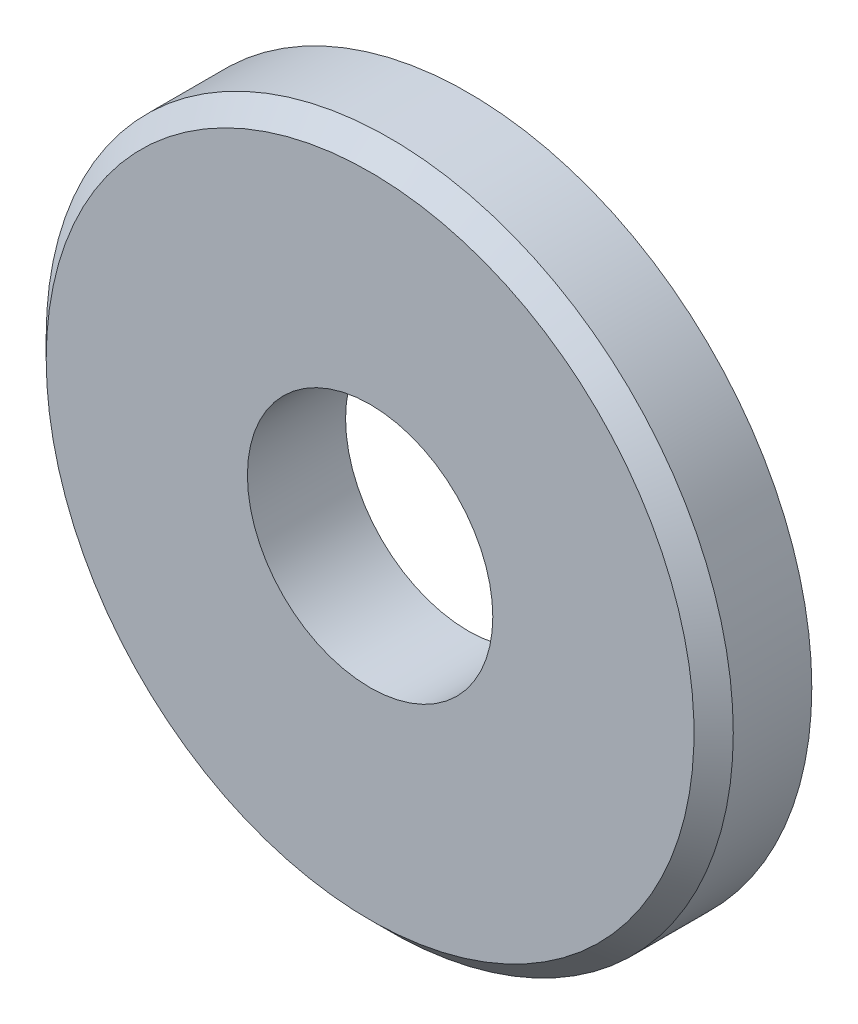
from build123d import *


with BuildPart() as part:
    # 草图1 → 旋转1 (revolve)
    with BuildSketch(Plane.XZ, mode=Mode.PRIVATE) as revolve_1_sk:
        Polygon((6.25, 2.5), (6.25, -2.5), (17.5, -2.5), (17.5, 1.5), (16.5, 2.5), align=None)
    revolve(revolve_1_sk.sketch.rotate(Axis((0, 0, 2.5), (0, 0, -1)), 180), axis=Axis((0, 0, 2.5), (0, 0, -1)))


solid = part.part
